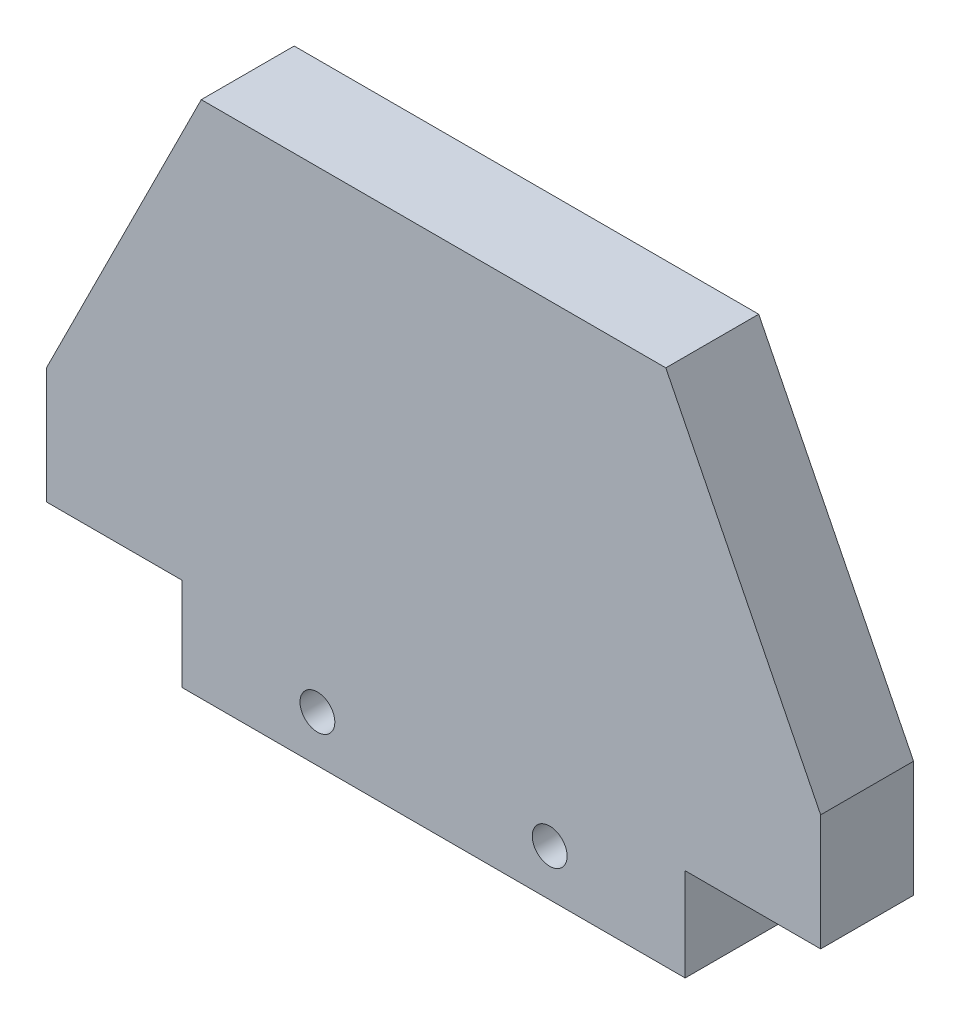
from build123d import *

# Parameters (mm, degrees)
SKETCH1_W                                           = 100
SKETCH1_H                                           = 55
BOSS_EXTRUDE1_DEPTH                                 = 12
SKETCH2_W                                           = 65
SKETCH2_H                                           = 12
BOSS_EXTRUDE2_DEPTH                                 = 12
CBORE_FOR_M4_HEX_SOCKET_HEAD_CAP_SCREW1_D           = 4.5
CBORE_FOR_M4_HEX_SOCKET_HEAD_CAP_SCREW1_CBORE_D     = 8
CBORE_FOR_M4_HEX_SOCKET_HEAD_CAP_SCREW1_CBORE_DEPTH = 4.4
CHAMFER1_SIZE                                       = 40
CHAMFER1_SIZE2                                      = 20
CHAMFER2_SIZE                                       = 20
CHAMFER2_SIZE2                                      = 40


with BuildPart() as part:
    # Sketch1 → Boss-Extrude1 (new body)
    with BuildSketch(Plane.XY):
        Rectangle(SKETCH1_W, SKETCH1_H)
    extrude(amount=BOSS_EXTRUDE1_DEPTH)

    # Sketch2 → Boss-Extrude2 (add)
    with BuildSketch(Plane.XZ.offset(27.5)):
        with Locations((0, 6)):
            Rectangle(SKETCH2_W, SKETCH2_H)
    extrude(amount=BOSS_EXTRUDE2_DEPTH)

    # CBORE for M4 Hex Socket Head Cap Screw1 (through all)
    with Locations(Plane(origin=(0, 0, 0), x_dir=(-1, 0, 0), z_dir=(0, 0, -1))):
        with Locations((15, -33.5), (-15, -33.5)):
            CounterBoreHole(CBORE_FOR_M4_HEX_SOCKET_HEAD_CAP_SCREW1_D / 2, CBORE_FOR_M4_HEX_SOCKET_HEAD_CAP_SCREW1_CBORE_D / 2, CBORE_FOR_M4_HEX_SOCKET_HEAD_CAP_SCREW1_CBORE_DEPTH)

    # Chamfer1
    chamfer1_edges = [part.edges().sort_by_distance(p)[0] for p in [
        (50, 27.5, 6),
    ]]
    chamfer1_side = [part.faces().sort_by_distance(p)[0] for p in [
        (50, 0, 6),
    ]]
    chamfer(chamfer1_edges, length=CHAMFER1_SIZE, length2=CHAMFER1_SIZE2, reference=chamfer1_side[0])

    # Chamfer2
    chamfer2_edges = [part.edges().sort_by_distance(p)[0] for p in [
        (-50, 27.5, 6),
    ]]
    chamfer2_side = [part.faces().sort_by_distance(p)[0] for p in [
        (-10, 27.5, 6),
    ]]
    chamfer(chamfer2_edges, length=CHAMFER2_SIZE, length2=CHAMFER2_SIZE2, reference=chamfer2_side[0])


solid = part.part
